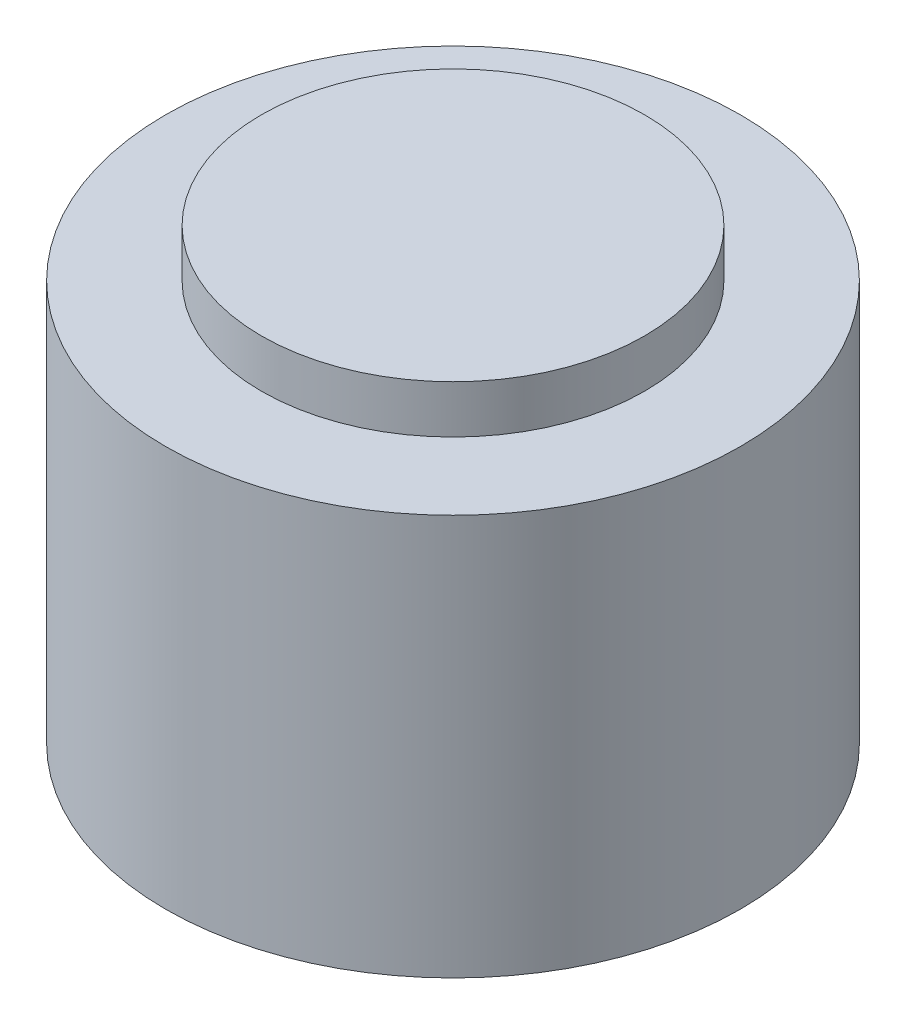
from build123d import *

# Parameters (mm, degrees)
SKETCH_1_R      = 18
EXTRUDE_1_DEPTH = 25.1
SKETCH_2_R      = 12
EXTRUDE_2_DEPTH = 3


with BuildPart() as part:
    # 草图1 → 凸台-拉伸1 (new body)
    with BuildSketch(Plane(origin=(0, 0, 0), x_dir=(1, 0, 0), z_dir=(0, 1, 0))):
        with Locations(Location((0, 0, 0), (0, 0, 270))):
            Circle(SKETCH_1_R)
    extrude(amount=EXTRUDE_1_DEPTH)

    # 草图2 → 凸台-拉伸2 (add)
    with BuildSketch(Plane(origin=(0, 25.1, 0), x_dir=(1, 0, 0), z_dir=(0, 1, 0))):
        with Locations(Location((0, 0, 0), (0, 0, 270))):
            Circle(SKETCH_2_R)
    extrude(amount=EXTRUDE_2_DEPTH)


solid = part.part
